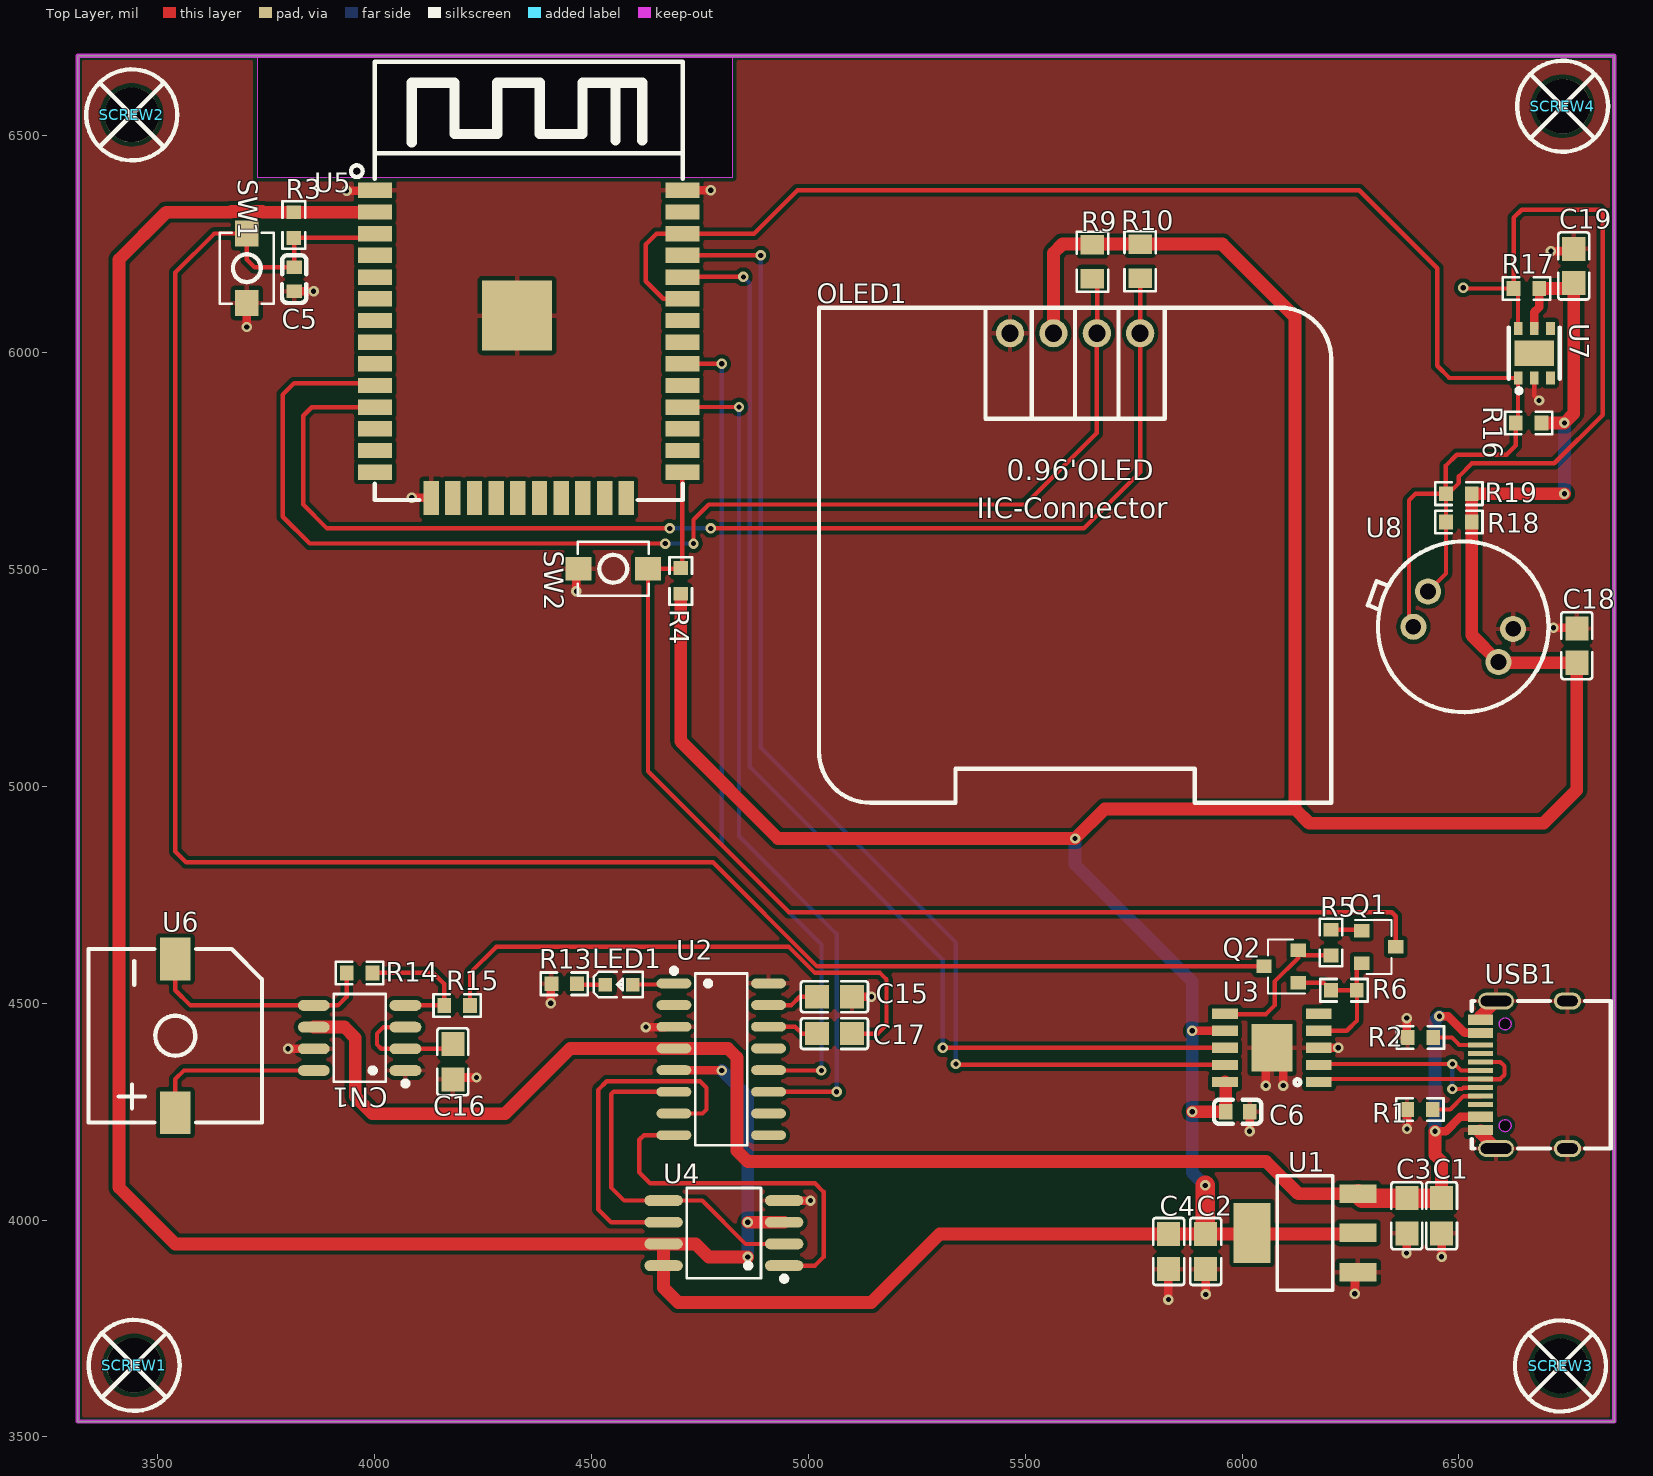
[diagram p0: Top Layer view]
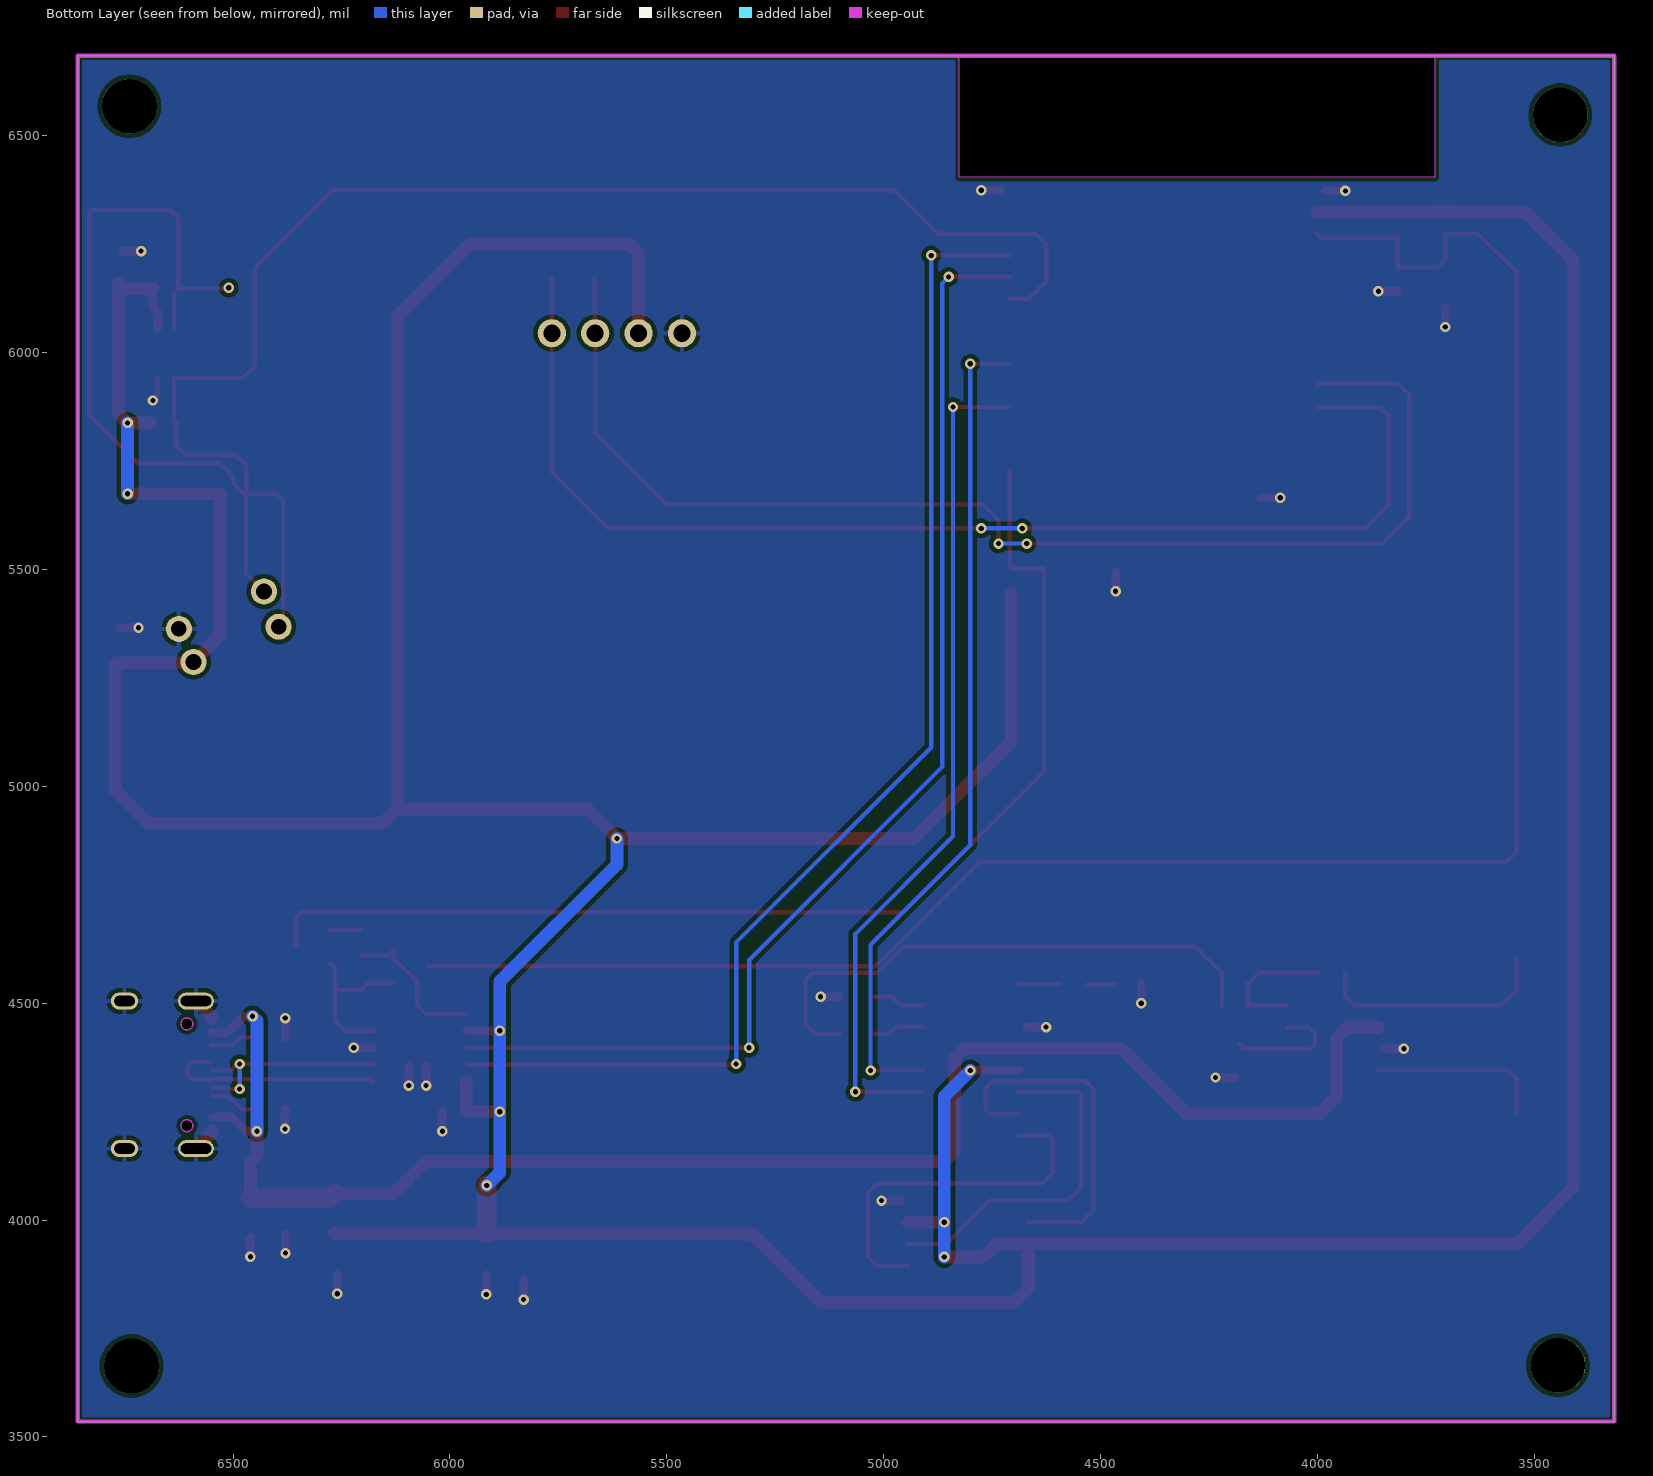
[diagram p1: Bottom Layer view, seen from below]
# Altium PCB MISC50923.pcbdoc
Units mil, origin at the board's own origin, x right, y up, seen from the top; angles counter-clockwise.
Board outline 3543.31 x 3149.61 mil, 2 copper layers (Top Layer, Bottom Layer), stack 62.206 mil thick; 46 components, 46 nets, 187 pads, 52 vias.

## Layer stack, top to bottom
Top Solder Mask Layer: solder mask 0.394, Dk 3.3
Top Layer: signal copper 1.379
Dielectric1: surface 59.449, FR4, Dk 4.5
Bottom Layer: signal copper 1.378
Bottom Solder Mask Layer: solder mask 0.394, Dk 3.3

## Board outline
3315,6685 3315,3535.39 6858.31,3535.39 6858.31,6685
cut-out: 3728.64,6685 3728.64,6405 4825,6405 4825,6685

## Design rules (kind name [scope] priority, off if disabled: settings)
BoardOutlineClearance copperThickness2oz_1 [All] p2 off: genericclearance=7.99 ignorepadtopadclearanceinfootprint=FALSE except(0: Arc-SplitContinuation Track-SplitContinuation SMDPad-SplitContinuation THPad-SplitContinuation Via-SplitContinuation Fill-SplitContinuation Region-SplitContinuation Poly-SplitContinuation Text-SplitContinuation Hole-SplitContinuation; 5.98: Arc-CutoutEdge SMDPad-CutoutEdge THPad-CutoutEdge Via-CutoutEdge Fill-CutoutEdge Region-CutoutEdge Text-CutoutEdge; 6.93: Hole-OutlineEdge Hole-CutoutEdge; 10: Poly-OutlineEdge Poly-CutoutEdge; 11.81: Arc-OutlineEdge Track-OutlineEdge SMDPad-OutlineEdge THPad-OutlineEdge Via-OutlineEdge Fill-OutlineEdge Region-OutlineEdge Text-OutlineEdge Track-CutoutEdge)
BoardOutlineClearance Plane_innerPlane_1 [All] p4 off: genericclearance=4.02 ignorepadtopadclearanceinfootprint=FALSE except(0: Arc-SplitContinuation Track-SplitContinuation SMDPad-SplitContinuation THPad-SplitContinuation Via-SplitContinuation Fill-SplitContinuation Region-SplitContinuation Poly-SplitContinuation Text-SplitContinuation Hole-SplitContinuation; 6: SMDPad-CutoutEdge THPad-CutoutEdge Via-CutoutEdge Fill-CutoutEdge Region-CutoutEdge Text-CutoutEdge; 6.93: Hole-OutlineEdge Hole-CutoutEdge; 10: Poly-OutlineEdge Poly-CutoutEdge; 11.8: Arc-OutlineEdge Track-OutlineEdge SMDPad-OutlineEdge THPad-OutlineEdge Via-OutlineEdge Fill-OutlineEdge Region-OutlineEdge Text-OutlineEdge; 11.81: Arc-CutoutEdge Track-CutoutEdge)
BoardOutlineClearance Copper_copperRegion_1 [All] p6 off: genericclearance=4.02 ignorepadtopadclearanceinfootprint=FALSE except(0: Arc-SplitContinuation Track-SplitContinuation SMDPad-SplitContinuation THPad-SplitContinuation Via-SplitContinuation Fill-SplitContinuation Region-SplitContinuation Poly-SplitContinuation Text-SplitContinuation Hole-SplitContinuation; 6: SMDPad-CutoutEdge THPad-CutoutEdge Via-CutoutEdge Fill-CutoutEdge Region-CutoutEdge Text-CutoutEdge; 6.93: Hole-OutlineEdge Hole-CutoutEdge; 10: Poly-OutlineEdge Poly-CutoutEdge; 11.8: Arc-OutlineEdge Track-OutlineEdge SMDPad-OutlineEdge THPad-OutlineEdge Via-OutlineEdge Fill-OutlineEdge Region-OutlineEdge Text-OutlineEdge; 11.81: Arc-CutoutEdge Track-CutoutEdge)
BoardOutlineClearance copperThickness1oz_1 [All] p8: genericclearance=4.02 ignorepadtopadclearanceinfootprint=FALSE except(0: Arc-SplitContinuation Track-SplitContinuation SMDPad-SplitContinuation THPad-SplitContinuation Via-SplitContinuation Fill-SplitContinuation Region-SplitContinuation Poly-SplitContinuation Text-SplitContinuation Hole-SplitContinuation; 6: SMDPad-CutoutEdge THPad-CutoutEdge Via-CutoutEdge Fill-CutoutEdge Region-CutoutEdge Text-CutoutEdge; 6.93: Hole-OutlineEdge Hole-CutoutEdge; 10: Poly-OutlineEdge Poly-CutoutEdge; 11.8: Arc-OutlineEdge Track-OutlineEdge SMDPad-OutlineEdge THPad-OutlineEdge Via-OutlineEdge Fill-OutlineEdge Region-OutlineEdge Text-OutlineEdge; 11.81: Arc-CutoutEdge Track-CutoutEdge)
Clearance copperThickness2oz [All] p1 off: gap=7.99 ignorepadtopadclearanceinfootprint=FALSE except(5.98: SMDPad-Track SMDPad-SMDPad THPad-Track SMDPad-THPad THPad-THPad Track-Via SMDPad-Via THPad-Via Via-Via Fill-Track Region-Track Fill-SMDPad Region-SMDPad Fill-THPad Region-THPad Fill-Via Region-Via Fill-Fill Fill-Region Region-Region Arc-Track Arc-SMDPad Arc-THPad Arc-Via Fill-Arc Region-Arc Arc-Arc Text-Track SMDPad-Text Text-THPad Text-Via Fill-Text Region-Text Arc-Text Text-Text; 6.93: Hole-Track Hole-SMDPad Hole-THPad Hole-Via Fill-Hole Region-Hole Hole-Arc Hole-Text; 10: Poly-Track Poly-SMDPad Poly-THPad Poly-Via Poly-Fill Poly-Region Poly-Poly Poly-Arc Poly-Text Poly-Hole)
Clearance Plane_innerPlane [All] p3 off: gap=4.02 ignorepadtopadclearanceinfootprint=FALSE except(5.98: SMDPad-Track SMDPad-SMDPad THPad-Track SMDPad-THPad THPad-THPad Track-Via SMDPad-Via THPad-Via Via-Via Fill-Track Region-Track Fill-SMDPad Region-SMDPad Fill-THPad Region-THPad Fill-Via Region-Via Fill-Fill Fill-Region Region-Region; 6: Arc-Track Arc-SMDPad Arc-THPad Arc-Via Fill-Arc Region-Arc Arc-Arc Text-Track SMDPad-Text Text-THPad Text-Via Fill-Text Region-Text Arc-Text Text-Text; 6.93: Hole-Track Hole-SMDPad Hole-THPad Hole-Via Fill-Hole Region-Hole Hole-Arc Hole-Text; 10: Poly-Track Poly-SMDPad Poly-THPad Poly-Via Poly-Fill Poly-Region Poly-Poly Poly-Arc Poly-Text Poly-Hole)
Clearance Copper_copperRegion [All] p5 off: gap=4.02 ignorepadtopadclearanceinfootprint=FALSE except(5.98: SMDPad-Track SMDPad-SMDPad THPad-Track SMDPad-THPad THPad-THPad Track-Via SMDPad-Via THPad-Via Via-Via Fill-Track Region-Track Fill-SMDPad Region-SMDPad Fill-THPad Region-THPad Fill-Via Region-Via Fill-Fill Fill-Region Region-Region; 6: Arc-Track Arc-SMDPad Arc-THPad Arc-Via Fill-Arc Region-Arc Arc-Arc Text-Track SMDPad-Text Text-THPad Text-Via Fill-Text Region-Text Arc-Text Text-Text; 6.93: Hole-Track Hole-SMDPad Hole-THPad Hole-Via Fill-Hole Region-Hole Hole-Arc Hole-Text; 10: Poly-Track Poly-SMDPad Poly-THPad Poly-Via Poly-Fill Poly-Region Poly-Poly Poly-Arc Poly-Text Poly-Hole)
Clearance copperThickness1oz [All] p7: gap=4.02 ignorepadtopadclearanceinfootprint=FALSE except(5.98: SMDPad-Track SMDPad-SMDPad THPad-Track SMDPad-THPad THPad-THPad Track-Via SMDPad-Via THPad-Via Via-Via Fill-Track Region-Track Fill-SMDPad Region-SMDPad Fill-THPad Region-THPad Fill-Via Region-Via Fill-Fill Fill-Region Region-Region; 6: Arc-Track Arc-SMDPad Arc-THPad Arc-Via Fill-Arc Region-Arc Arc-Arc Text-Track SMDPad-Text Text-THPad Text-Via Fill-Text Region-Text Arc-Text Text-Text; 6.93: Hole-Track Hole-SMDPad Hole-THPad Hole-Via Fill-Hole Region-Hole Hole-Arc Hole-Text; 10: Poly-Track Poly-SMDPad Poly-THPad Poly-Via Poly-Fill Poly-Region Poly-Poly Poly-Arc Poly-Text Poly-Hole)
DiffPairsRouting differentialPair [All] p1: maxlimit=6 minlimit=6 mostfreqgap=6 toplayer_minwidth=5 toplayer_prefwidth=10 toplayer_maxwidth=100 toplayer_mingap=6 toplayer_prefgap=6 toplayer_maxgap=6 bottomlayer_minwidth=5 bottomlayer_prefwidth=10 bottomlayer_maxwidth=100 bottomlayer_mingap=6 bottomlayer_prefgap=6 bottomlayer_maxgap=6 maxuncoupledlength=10
HoleToHoleClearance otherClearance [All] p1: gap=11.81 allowstackedmicrovias=TRUE
Length netLength [All] p1: minlimit=0 maxlimit=0
PasteMaskExpansion pasteMaskExpansion [All] p1: expansion=0
PlaneConnect innerPlane [All] p1: planeconnectstyle=Relief reliefexpansion=20 reliefentries=4 reliefconductorwidth=10 reliefairgap=10
PolygonConnect copperRegion [All] p1: connectstyle=Relief reliefconductorwidth=10 reliefentries=4 polygonreliefangle="90 Angle" airgapwidth=10 via.connectstyle=Relief via.reliefconductorwidth=10 via.reliefentries=4 via.polygonreliefangle="90 Angle" via.airgapwidth=10
RoutingVias viaSize [All] p1: holewidth=12.01 width=24.02 viastyle="Through Hole" minholewidth=11.81 minwidth=19.68 maxholewidth=248.03 maxwidth=393.7
SolderMaskExpansion solderMaskExpansion [IsVia] p1: expansion=-1000 istentingtop=TRUE
SolderMaskExpansion solderMaskExpansion [All] p2: expansion=2 istentingtop=FALSE
Width copperThickness2oz_2 [All] p1 off: maxlimit=100 minlimit=8 preferedwidth=10
Width copperThickness1oz_2 [All] p2: maxlimit=100 minlimit=5 preferedwidth=10

## Components (designator, comment, footprint, x,y, rotation, side; value= is the part's Value field where it differs from the comment)
C1 "10u" C0805 6460,4010 r90 top
C2 "10u" C0805 5916.16,3927.49 r90 top
C3 "104" C0805 6380,4010 r90 top
C4 "104" C0805 5830.86,3927.49 r90 top
C5 "1uF" C0603 3814.11,6169.56 r270 top
C6 "100nF" C0603_1 5989.84,4249.8 r180 top
C15 "104" C0805 5060,4515 r180 top
C16 "105" C0805 4180,4365 r270 top
C17 "105" C0805 5060,4430 r180 top
C18 "22uF" C0805_1 6771.89,5324.62 r270 top
C19 "100nF" C0805_1 6764.87,6200.18 r270 top
CN1 "AD8002D" SOP-8_L5.0-W3.8-P1.27-LS6.0-BL 3965,4420 r90 top
LED1 "" LED_0603 4565.31,4543.25 r0 top
OLED1 "" 0.96OLED_4P 5615,6045 r0 top
Q1 "S8050" SOT-23 6315,4630 r0 top
Q2 "S8050" SOT-23 6090,4585 r180 top
R1 "5.1kΩ" R0603 6410,4255 r180 top
R2 "5.1kΩ" R0603 6411.14,4420.99 r180 top
R3 "10kΩ" R0603 3813.27,6294.56 r90 top
R4 "10kΩ" R0603 4705.61,5473.74 r270 top
R5 "4.7kΩ" R0603 6205,4640 r90 top
R6 "4.7kΩ" R0603 6235,4530 r180 top
R9 "4.7K" R0805 5655,6210 r270 top
R10 "4.7K" R0805 5765,6211.26 r270 top
R13 "100R" R0603 4436.96,4545.01 r0 top
R14 "47K" R0603 3965,4570 r180 top
R15 "20K" R0603 4190,4495 r180 top
R16 "4.7K" R0603 6660.88,5838.28 r0 top
R17 "4.7K" R0603 6655.88,6148.28 r0 top
R18 "1.6K" R0603 6500,5610 r0 top
R19 "1.6K" R0603 6500,5675 r0 top
SCREW1 "" M3螺丝 3445,3665 r0 top
SCREW2 "" M3螺丝 3439.68,6548.54 r0 top
SCREW3 "" M3螺丝 6734.37,3663.54 r0 top
SCREW4 "" M3螺丝 6739.06,6568.54 r0 top
SW1 "" Key_SMD_3x4x2 3705,6195 r270 top
SW2 "" Key_SMD_3x4x2 4549.97,5501.86 r180 top
U1 "AMS1117-3.3" SOT-223_L6.5-W3.5-P2.30-LS7.0-BR 6145,3970 r0 top
U2 "JQ8400-FN" SOP-16_L9.9-W3.9-P1.27-LS6.0-BL 4798.97,4370.77 r270 top
U3 "CH340K" ESOP-10_L4.9-W3.9-P1.00-LS6.2-BL-EP 6068.92,4397.2 r90 top
U4 "W25Q128JVSIQ" SOIC-8_L5.3-W5.3-P1.27-LS8.0-BL 4805,3970 r90 top
U5 "2.4GHz" WIFIM-SMD_ESP32-WROOM-32-N4 4355,6020 r0 top
U6 "SPK-HN9650B" BUZ-SMD_L9.6-W9.6-LS10.0-R 3540,4425 r270 top
U7 "SHT20-TR-1.5KS" DFN-6_L3.0-W3.0-P0.95-TR-EP 6673.83,5999.05 r180 top
U8 "MLX90640ESF-BAA-000-TU" TO-39_4P-BD9.3_MLX90640ESF-BAA-000-TU_H5.7 6510,5368.15 r0 top
USB1 "" USB-C-SMD_TYPEC-304-BCP16 6650,4335 r90 top

## Footprints (in the part's own frame and the unit in brackets; to place one, negate y for a bottom-side part, rotate by r counter-clockwise, add the part's x,y. Pads: shape width x height; smd on the part's side, far side on the other; paste and mask are expansions set on the pad)
0.96OLED_4P [mm]
  round 1.65 hole 1 copper offset 0,0: 1(-3.81,-0.001) 2(-1.27,0.002) 3(1.27,0.002) 4(3.81,0.002)
  silkscreen extent -15,-27.5 15,1.5
BUZ-SMD_L9.6-W9.6-LS10.0-R [mm]
  rect 2.5x1.8 smd: 1(4.5,0) 2(-4.5,0)
  silkscreen extent -5.08,-5.08 5.08,5.08
C0603 [mm]
  rect 0.8x0.9 smd: 1(-0.7,0) 2(0.7,0)
  silkscreen extent -1.41,-0.71 1.39,0.72
C0603_1 [mm]
  rect 0.8x0.9 smd: 1(-0.7,0) 2(0.7,0)
  silkscreen extent -1.39,-0.71 1.39,0.71
C0805 [mm]
  rect 1.41x1.35 smd paste-100 mask+0.051: 1(-1.03,0) 2(1.03,0)
  silkscreen extent -1.96,-0.9 1.96,0.9
C0805_1 [mm]
  rect 1.41x1.35 smd paste-100 mask+0.051: 1(-1,0) 2(1,0)
  silkscreen extent -1.96,-0.9 1.96,0.9
DFN-6_L3.0-W3.0-P0.95-TR-EP [mm]
  rect 0.5x0.75 smd: 1(0.95,1.452) 2(0,1.451) 3(-0.95,1.45) 4(-0.95,-1.451) 5(0,-1.452) 6(0.95,-1.451)
  rect 2.3x1.5 smd: 7(0.004,-0.001)
  silkscreen extent -1.5,-1.5 1.5,2.34
ESOP-10_L4.9-W3.9-P1.00-LS6.2-BL-EP [mm]
  rect 0.6x1.5 smd: 1(-2,-2.75) 2(-1,-2.75) 3(0,-2.75) 4(1,-2.75) 5(2,-2.75) 6(2,2.75) 7(1,2.75) 8(0,2.75) 9(-1,2.75) 10(-2,2.75)
  rect 2.8x2.4 smd: 11(0,0)
  silkscreen extent -2.18,-1.66 -1.84,-1.32
Key_SMD_3x4x2 [mm]
  rect 1.53x1.36 smd paste+0 mask+0.051: 1(-2.035,0) 2(2.035,0)
  silkscreen extent -2.08,-1.58 2.08,1.58
LED_0603 [mil]
  rect 31.5x31.5 smd paste+0 mask+2: 1(-33.5,-0.4) 2(29.5,-0.2)
  silkscreen extent -61,-30 53,30
M3螺丝 [mil]
  round 126 hole 126 paste+0 mask+4: 1(0,0)
  silkscreen extent -105,-105 105,105
R0603 [mil]
  rect 31.75x34.02 smd paste-3937.01 mask+2: 1(-29.66,0) 2(29.66,0)
  silkscreen extent -55,-26 55,26
R0805 [mm]
  rect 1.133x1.377 smd paste-100 mask+0.051: 1(-1,0) 2(1,0)
  silkscreen extent -1.76,-0.92 1.76,0.92
SOIC-8_L5.3-W5.3-P1.27-LS8.0-BL [mm]
  oval 0.63x2.25 smd: 1(-1.905,-3.53) 2(-0.635,-3.53) 3(0.635,-3.53) 4(1.905,-3.53) 5(1.905,3.53) 6(0.635,3.53) 7(-0.635,3.53) 8(-1.905,3.53)
  silkscreen extent -2.82,-3.68 2.64,2.18
SOP-8_L5.0-W3.8-P1.27-LS6.0-BL [mm]
  oval 0.63x1.865 smd: 1(-1.905,-2.682) 2(-0.635,-2.682) 3(0.635,-2.682) 4(1.905,-2.682) 5(1.905,2.682) 6(0.635,2.682) 7(-0.635,2.682) 8(-1.905,2.682)
  silkscreen extent -2.82,-2.83 2.58,1.52
SOP-16_L9.9-W3.9-P1.27-LS6.0-BL [mil]
  oval 22.6x80.24 smd: 1(-175,-109.02) 2(-125,-109.02) 3(-75,-109.02) 4(-25,-109.02) 5(25,-109.02) 6(75,-109.02) 7(125,-109.02) 8(175,-109.02) 9(175,109.02) 10(125,109.02) 11(75,109.02) 12(25,109.02) 13(-25,109.02) 14(-75,109.02) 15(-125,109.02) 16(-175,109.02)
  silkscreen extent -210,-115 198,60
SOT-23 [mm]
  rect 0.9x0.8 smd paste+0 mask+0.102: 1(-1,0.95) 2(-1,-0.95) 3(1,0)
  silkscreen extent -1.4,-1.58 0.76,1.58
SOT-223_L6.5-W3.5-P2.30-LS7.0-BR [mil]
  rect 85x43 smd paste+0 mask+4: 1(122,-90.5) 2(122,0.5) 3(122,90.5)
  rect 85x138 smd paste+0 mask+4: 4(-122,0.5)
  silkscreen extent -64,-132 64,132
TO-39_4P-BD9.3_MLX90640ESF-BAA-000-TU_H5.7 [mil]
  round 60 hole 36: 1(-114.96,0) 2(81.29,-81.29) 3(114.96,-5) 4(-81.3,81.3)
  silkscreen extent -220,-197 197,197
USB-C-SMD_TYPEC-304-BCP16 [mil]
  oval 39.4x82.7 hole 23.6 slot 70.9 at 90 deg paste+0 mask+2: 13(-170.1,64.3) 14(170.1,64.3)
  oval 39.4x63 hole 23.6 slot 47.2 at 90 deg paste+0 mask+2: 15(-170.1,-100.3) 16(170.1,-100.3)
  rect 23.6x57.1 smd paste+0 mask+2: A1B12(-127,100.3) A4B9(-96.5,100.3) B1A12(126.8,100.3) B4A9(96.5,100.3)
  rect 11.8x57.1 smd paste+0 mask+2: A5(-49.2,100.3) A6(-9.8,100.3) A7(9.8,100.3) A8(49.2,100.3) B5(68.9,100.3) B6(29.5,100.3) B7(-29.5,100.3) B8(-68.9,100.3)
  Board Outline Layer circle w0.1: c117.3,43.4 r13.8
  Board Outline Layer circle w0.1: c-117.3,43.4 r13.8
  Board Outline Layer region: 117.3,29.6 111.31,30.97 106.51,34.8 103.85,40.33 103.85,46.47 106.51,52 111.31,55.83 117.3,57.2 117.3,57.2 123.29,55.83 128.09,52 130.75,46.47 130.75,40.33 128.09,34.8 123.29,30.97 117.3,29.6
  Board Outline Layer region: 117.3,29.6 114.23,29.95 111.31,30.97 108.7,32.61 106.51,34.8 104.87,37.41 103.85,40.33 103.5,43.4 103.85,46.47 104.87,49.39 106.51,52 108.7,54.19 111.31,55.83 114.23,56.85 117.3,57.2 120.37,56.85 123.29,55.83 125.9,54.19 128.09,52 129.73,49.39 130.75,46.47 131.1,43.4 130.75,40.33 129.73,37.41 128.09,34.8 125.9,32.61 123.29,30.97 120.37,29.95
  Board Outline Layer region: -117.3,29.6 -123.29,30.97 -128.09,34.8 -130.75,40.33 -130.75,46.47 -128.09,52 -123.29,55.83 -117.3,57.2 -117.3,57.2 -111.31,55.83 -106.51,52 -103.85,46.47 -103.85,40.33 -106.51,34.8 -111.31,30.97 -117.3,29.6
  Board Outline Layer region: -117.3,29.6 -120.37,29.95 -123.29,30.97 -125.9,32.61 -128.09,34.8 -129.73,37.41 -130.75,40.33 -131.1,43.4 -130.75,46.47 -129.73,49.39 -128.09,52 -125.9,54.19 -123.29,55.83 -120.37,56.85 -117.3,57.2 -114.23,56.85 -111.31,55.83 -108.7,54.19 -106.51,52 -104.87,49.39 -103.85,46.47 -103.5,43.4 -103.85,40.33 -104.87,37.41 -106.51,34.8 -108.7,32.61 -111.31,30.97 -114.23,29.95
  Multi-Layer board cut-out: 117.3,29.6 111.31,30.97 106.51,34.8 103.85,40.33 103.85,46.47 106.51,52 111.31,55.83 117.3,57.2 117.3,57.2 123.29,55.83 128.09,52 130.75,46.47 130.75,40.33 128.09,34.8 123.29,30.97 117.3,29.6
  Multi-Layer board cut-out: -117.3,29.6 -123.29,30.97 -128.09,34.8 -130.75,40.33 -130.75,46.47 -128.09,52 -123.29,55.83 -117.3,57.2 -117.3,57.2 -111.31,55.83 -106.51,52 -103.85,46.47 -103.85,40.33 -106.51,34.8 -111.31,30.97 -117.3,29.6
  silkscreen extent -170,-200 170,120
WIFIM-SMD_ESP32-WROOM-32-N4 [mm]
  rect 2x0.9 smd paste+0 mask+0.05: 1(-9,9.005) 2(-9,7.735) 3(-9,6.465) 4(-9,5.195) 5(-9,3.925) 6(-9,2.655) 7(-9,1.385) 8(-9,0.115) 9(-9,-1.155) 10(-9,-2.425) 11(-9,-3.695) 12(-9,-4.965) 13(-9,-6.235) 14(-9,-7.505) 25(9,-7.505) 26(9,-6.235) 27(9,-4.965) 28(9,-3.695) 29(9,-2.425) 30(9,-1.155) 31(9,0.115) 32(9,1.385) 33(9,2.655) 34(9,3.925) 35(9,5.195) 36(9,6.465) 37(9,7.735) 38(9,9.005)
  rect 0.9x2 smd paste+0 mask+0.05: 15(-5.715,-9.005) 16(-4.445,-9.005) 17(-3.175,-9.005) 18(-1.905,-9.005) 19(-0.635,-9.005) 20(0.635,-9.005) 21(1.905,-9.005) 22(3.175,-9.005) 23(4.445,-9.005) 24(5.715,-9.005)
  rect 4.1x4.1 smd paste+0 mask+0.05: 39(-0.68,1.665)
  silkscreen extent -10.41,-9.13 9.02,16.54

## Via types
v1: diameter 24.02, hole 12, Top Layer to Bottom Layer, 52 vias

## Nets (pads, with @x,y where several pads share a name; then routed paths per layer and width w, separated by ;. In a path a pad name is that pad's centre, name@x,y a point inside that pad or via, vN(x,y) a via of type N, cw(c..) or ccw(c..) an arc to the next point about the centre after c; other vN are vias at no path point)
3V3: C2.2 C4.2 C6.2 C18.2 C19.2 OLED1.2 R3.2 R4.2 R9.1 R10.1 R16.2 R17.2 R18.2 R19.2 U1.2 U1.4 U2.5 U3.7 U3.10 U4.3 U4.7 U4.8 U5.2 U7.5 U8.2 | length 14342.9
  Top Layer w19.68: U2.5 4690.71,4345 v1(4800,4345) ; v1(5885,4436.57) U3.7 ; U7.5 6673.83,6093.83 6685.54,6105.54 R17.2
  Top Layer w29.53: U5.2 4000.36,6324.22 R3.2 3742.13,6324.22 3740.37,6325.99 3669.63,6325.99 3667.87,6324.22 3519.22,6324.22 3410,6215 3410,4075 3540,3945 U4.7 ; R4.2 4705.61,5104.39 4930,4880 v1(5615,4880) 5683.16,4948.16 6121.84,4948.16 ; v1(4860,3915) 4770,3915 4740,3945 U4.7 ; v1(4860,3995) U4.3 ; v1(5885,4250) 5962.08,4250 C6.2 5962.28,4316.83 U3.10 ; 6121.84,4988.51 6121.84,4948.16 ; U1.2 6264.54,3968.04 C2.2 C4.2 5303.04,3968.04 5145,3810 4700,3810 4666.02,3843.98 U4.8 U4.7 ; R17.2 6752.34,6148.28 C19.2 6764.87,5859.87 v1(6743.28,5838.28) R16.2 ; v1(6743.28,5675) R19.2 R18.2 6529.66,5348.49 U8.2 6592.9,5285.25 C18.2 6771.89,4991.89 6695,4915 6155,4915 6121.84,4948.16
  Top Layer w30: OLED1.2@5565,6045.05 5565,6230 5585.63,6250.63 R10.1 5954.37,6250.63 6121.84,6083.16 6121.84,4988.51
  Top Layer w45: v1(5915,4080) 5915,3969.2 C2.2
  Bottom Layer w29.53: v1(4800,4345) 4860,4285 v1(4860,3995) v1(4860,3915) ; v1(5615,4880) 5615,4820 5885,4550 v1(5885,4436.57) v1(5885,4250) 5885,4110 v1(5915,4080) ; v1(6743.28,5675) v1(6743.28,5838.28)
5V: C1.2 C3.2 CN1.6 U1.3 U2.4 USB1.A4B9 USB1.B4A9 | length 3753
  Top Layer w19.68: v1(6445,4205) 6470,4205 6503.5,4238.5 USB1.A4B9 ; v1(6455,4470) 6475,4470 6513.5,4431.5 USB1.B4A9
  Top Layer w29.53: CN1.6 3930,4445 3955,4420 3955,4285 3995,4245 4300,4245 4450.77,4395.77 U2.4 4814.23,4395.77 4835,4375 4835,4160 4860,4135 6055,4135 6129.5,4060.5 U1.3 ; v1(6445,4205) 6445,4150 6460,4135 C1.2
  Top Layer w45: U1.3 6276.95,4050.55 C3.2 C1.2
  Bottom Layer w29.53: v1(6445,4205) 6445,4460 v1(6455,4470)
$1N28: Q1.1 R5.2 | length 71.6
  Top Layer w10: R5.2 6273.37,4669.66 Q1.1
$1N115: OLED1.3 R9.2 U5.10 | length 2904.2
  Top Layer w10: U5.10 3995.2,5930 3814.43,5930 3787.93,5903.5 3787.93,5622.07 3850,5560 v1(4670,5560) ; v1(4735,5560) 4735,5615 4770,5650 5500,5650 5665,5815 5665,6045.05 5666.26,6046.31 R9.2@5666.26,6170.63
  Bottom Layer w10: v1(4670,5560) v1(4735,5560)
$1N125: C15.2 U2.15 | length 119.4
  Top Layer w10: U2.15 4960.77,4495.77 4980,4515 C15.2
$1N144: LED1.1 R13.2 | length 66.1
  Top Layer w10: R13.2 4468.78,4542.85 LED1.1
$1N146: C16.1 CN1.2 CN1.3 | length 280.3
  Top Layer w10: CN1.3 4020,4445 4005,4430 4005,4405 4015,4395 CN1.2 4169.45,4395 C16.1
$1N148: CN1.4 R14.1 R15.2 | length 315.6
  Top Layer w10: R14.1 4135,4570 4160.34,4544.66 R15.2 CN1.4
$1N149: C17.1 R15.1 | length 1283.8
  Top Layer w10: R15.1 4219.66,4569.66 4280,4630 4955,4630 5015,4570 5165,4570 5180,4555 5180,4450 5160,4430 C17.1
$1N151: CN1.5 R14.2 U6.2 | length 545.1
  Top Layer w10: U6.2 3540,4530 3575,4495 CN1.5 3915,4495 3935.34,4515.34 R14.2
$1N152: CN1.8 U6.1 | length 404.9
  Top Layer w10: U6.1 3540,4325 3560,4345 CN1.8
CC1: R1.1 USB1.A5 | length 122.8
  Top Layer w10: R1.1 6480,4255 6510.8,4285.8 USB1.A5
CC2: R2.1 USB1.B5 | length 116
  Top Layer w10: R2.1 6484.01,4420.99 6501.1,4403.9 USB1.B5
D+: U3.1 USB1.A6 USB1.B6 | length 514.1
  Top Layer w10: U3.1 6183.92,4325.2 USB1.A6 6549.9,4325 6595,4325 6605,4335 6605,4355 6595.5,4364.5 USB1.B6
D-: U3.2 USB1.A7 USB1.B7 | length 503.6
  Top Layer w10: U3.2 6179.35,4360 6489.71,4360 6504.91,4344.8 USB1.A7 ; v1(6485,4302.21) 6507.21,4302.21 6510.5,4305.5 USB1.B7
  Bottom Layer w10: v1(6485,4302.21) v1(6485,4360)
DTR: Q1.2 Q2.1 R6.1 R6.2 U3.4 | length 377.4
  Top Layer w10: Q2.1 6187.74,4547.6 R6.2 R6.1 ; U3.4 6241.57,4436.57 6265,4460 6265,4529.66 R6.1 ; Q1.2 6264.66,4581.63 R6.1
EN: C5.1 Q2.3 R3.1 SW1.1 U5.3 | length 4593.9
  Top Layer w10: U5.3 3991.04,6264.9 R3.1 3814.11,6264.06 C5.1 3722.88,6197.12 3705,6215 SW1.1 3630.12,6275.12 3540,6185 3540,4850 3565,4825 4780,4825 5020,4585 Q2.3
GND: C1.1 C2.1 C3.1 C4.1 C5.2 C6.1 C15.1 C16.2 C18.1 C19.1 CN1.1 CN1.7 OLED1.1 R1.2 R2.2 R13.1 SW1.2 SW2.2 U1.1 U2.3 U2.16 U3.3 U3.11 U4.4 U5.1 U5.15 U5.38 U5.39 U7.2 U8.3 USB1.13 USB1.14 USB1.15 USB1.16 USB1.A1B12 USB1.B1A12 | length 1288.6
  Top Layer w10: U7.2 6673.83,5901.17 v1(6685,5890)
  Top Layer w19.68: v1(3705,6059.38) SW1.2@3705,6104.19 ; v1(3800.2,4395) CN1.7@3845,4395 ; C5.2 v1(3858.91,6142) ; v1(3935,6373.18) U5.1@3979.8,6373.18 ; v1(4085.2,5665.47) U5.15 ; C16.2@4189.84,4328.78 v1(4234.65,4328.78) ; v1(4405.66,4500.21) R13.1@4405.66,4545.01 ; v1(4465,5450.2) SW2.2@4465,5495 ; v1(4625.2,4445) U2.3@4670,4445 ; U5.38@4730,6375 v1(4774.8,6375) ; U4.4@4960,4045 v1(5004.8,4045) ; C15.1 v1(5145.35,4515) ; v1(5830.07,3816.74) C4.1@5830.07,3861.54 ; v1(5916.16,3828.53) C2.1@5916.16,3873.33 ; v1(6017.4,4205) C6.1 ; v1(6055,4310.2) U3.11@6055,4355 ; v1(6095,4310.2) U3.11@6095,4355 ; U3.3 v1(6221.98,4397.2) ; v1(6260,3830.2) U1.1@6260,3875 ; v1(6379.21,3923.96) C3.1@6379.21,3968.76 ; R2.2@6379.84,4420.99 v1(6379.84,4465.8) ; v1(6380.34,4210.2) R1.2 ; v1(6460,3915.62) C1.1@6460,3960.42 ; v1(6712.19,6234.44) C19.1@6757,6234.44 ; v1(6718.11,5365.86) C18.1@6762.91,5365.86
  Top Layer w29.53: USB1.A1B12@6549.7,4205.95 6549.7,4200.9 USB1.13 ; USB1.B1A12@6549.7,4464.05 6549.7,4469.1 USB1.14
IO0: Q1.3 R4.1 SW2.1 U5.25 | length 2699.2
  Top Layer w10: U5.25 4709.33,5507.11 R4.1 4704.08,5501.86 SW2.1 4630.09,5034.91 4955,4710 6345,4710 6354.37,4700.63 Q1.3
IO2: U5.24
IO4: U5.26
IO5: U5.29
IO12: U5.14
IO13: U5.16
IO14: U5.13
IO16: U5.27
IO17: U2.11 U5.28 | length 1960.3
  Top Layer w10: U5.28 4709.8,5875 v1(4840,5875) ; U2.11 v1(5065,4295.77)
  Bottom Layer w10: v1(4840,5875) 4840,4885 5065,4660 v1(5065,4295.77)
IO18: U2.12 U5.30 | length 1937.8
  Top Layer w10: U5.30 v1(4800,5974.53) ; U2.12 4908.75,4345 v1(5030,4345)
  Bottom Layer w10: v1(4800,5974.53) 4800,4865 5030,4635 v1(5030,4345)
IO19: U5.31
IO21: R16.1 R17.1 R18.1 R19.1 U5.33 U5.36 U7.1 U7.6 U8.1 U8.4 | length 5096
  Top Layer w10: U5.33 4665.47,6124.53 4625,6165 4625,6250 4649.53,6274.53 U5.36 4874.53,6274.53 4975,6375 6270,6375 6450,6195 6450,5970 6478.12,5941.88 U7.1 6636.43,5843.49 R16.1 6631.22,5786.22 6610,5765 6495,5765 6470,5740 6470,5675.34 R19.1 6400,5675 6385,5660 6385,5378.19 U8.1 ; U8.4 6470.34,5491.09 R18.1 6470.34,5670.34 6500,5700 6500,5715 6530,5745 6720,5745 6832.07,5857.07 6832.07,6322.93 6825,6330 6645,6330 6626.22,6311.22 R17.1 ; v1(6510,6150) 6511.72,6148.28 R17.1 ; U7.6 6636.43,6138.07 R17.1
IO23: U5.37
IO26: OLED1.4 R10.2 U5.11 | length 2832.3
  Top Layer w10: U5.11 3854.53,5874.53 3835,5855 3835,5650 3890,5595 v1(4680,5595) ; v1(4775,5595) 5635,5595 5765,5725 5765,6045.05 R10.2
  Bottom Layer w10: v1(4680,5595) v1(4775,5595)
IO27: U5.12
IO32: U5.8
IO33: U5.9
IO34: U5.6
IO35: U5.7
JQ_BUSY: LED1.2 U2.1 | length 96.3
  Top Layer w10: LED1.2 4687.22,4543.05 U2.1
JQ_L: C17.2 U2.14 | length 118
  Top Layer w10: U2.14 4969.23,4445.77 4985,4430 C17.2
JQ_R: U2.13
RTS: Q2.2 R5.1 U3.6 | length 353.6
  Top Layer w10: U3.6 5961.59,4475 6055,4475 6075,4495 6075,4550 6129.37,4604.37 Q2.2 6141.43,4610.34 R5.1
SPI_CS: U2.8 U4.1 | length 852.3
  Top Layer w10: U2.8 4620.77,4195.77 4610,4185 4610,4110 4635,4085 5015,4085 5035,4065 5035,3915 5015,3895 U4.1
SPI_DIO: U2.6 U4.2 U4.5 | length 815.2
  Top Layer w10: U2.6 4550.77,4295.77 4545,4290 4545,4075 4575,4045 U4.5 4755,4045 4855,3945 U4.2
SPI_SCK: U2.7 U4.6 | length 831.8
  Top Layer w10: U4.6 4545,3995 4515,4025 4515,4300 4535,4320 4750,4320 4765,4305 4765,4255 4755.77,4245.77 U2.7
U0RX: U3.8 U5.34 | length 2759.9
  Top Layer w10: U5.34 4709.8,6175 v1(4850,6175) ; v1(5310,4397.2) U3.8
  Bottom Layer w10: v1(4850,6175) 4865,6160 4865,5045 5310,4600 v1(5310,4397.2)
U0TX: U3.9 U5.35 | length 2853.1
  Top Layer w10: U5.35 v1(4890,6224.53) ; v1(5340,4360) 5342.17,4357.83 U3.9
  Bottom Layer w10: v1(4890,6224.53) 4890,5090 5340,4640 v1(5340,4360)
pads on no net: SCREW1.1 SCREW2.1 SCREW3.1 SCREW4.1 U2.2 U2.9 U2.10 U3.5 U5.4 U5.5 U5.17 U5.18 U5.19 U5.20 U5.21 U5.22 U5.23 U5.32 U7.3 U7.4 U7.7 USB1.A8 USB1.B8

## Polygon pours and split planes (outlines as drawn)
GND on Top Layer (solid, remove dead copper, pour order 0): 3000,6920 3000,3000 7615,3000 7615,6920
GND on Bottom Layer (solid, remove dead copper, pour order 2): 3045,6845 3045,3070 7470,3070 7470,6845

## Keep-outs
Board Outline Layer:
  region: 3728.64,6685 3728.64,6405 4825,6405 4825,6685
  region: 3728.64,6685 3728.64,6405 4825,6405 4825,6685
  lines w0.1: 3728.64,6405 3728.64,6685 4825,6685 4825,6405 3728.64,6405
  lines w10: 3315,3535.39 3315,6685 6858.31,6685 6858.31,3535.39 3315,3535.39

## Silkscreen, mask and mechanical layers (free items; w line width, h text height)
Mechanical Layer:
  lines w0.1: 3728.64,6405 3728.64,6685 4825,6685 4825,6405 3728.64,6405